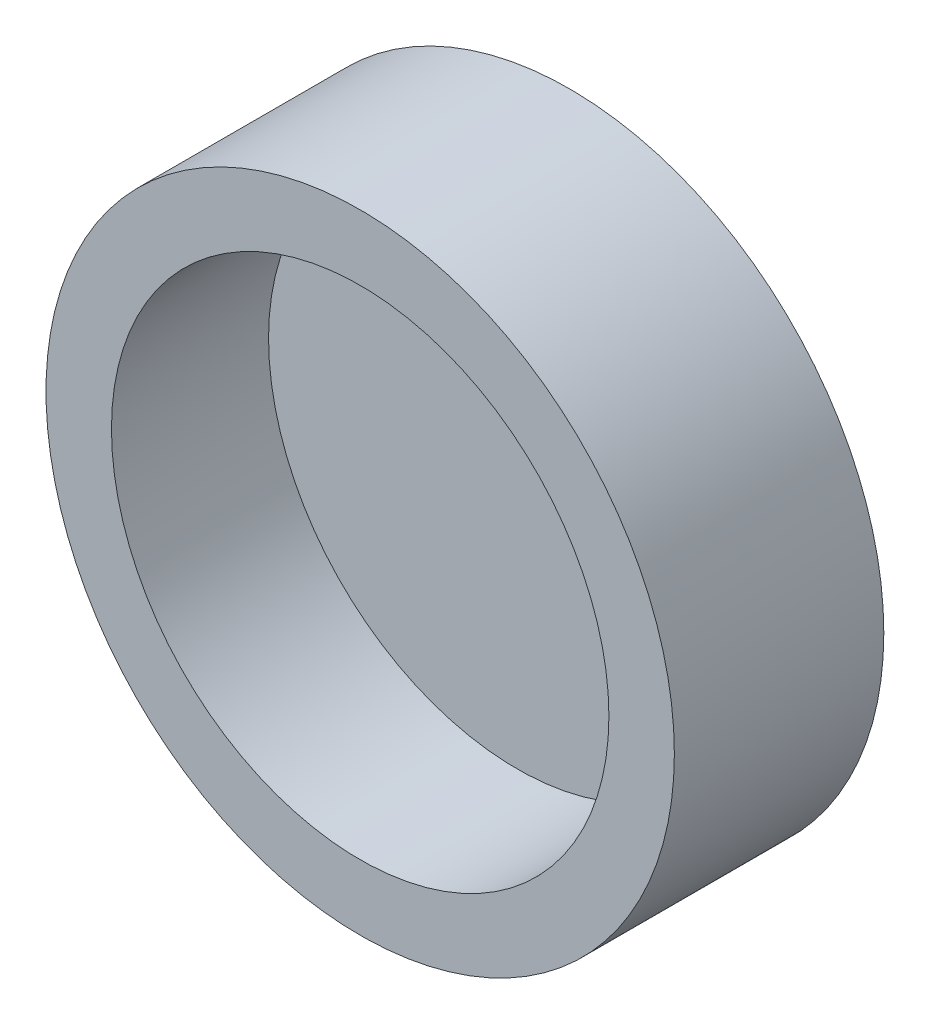
from build123d import *

# Parameters (mm, degrees)
SKETCH1_R           = 12
BOSS_EXTRUDE1_DEPTH = 8
SKETCH2_R           = 9.5
CUT_EXTRUDE1_DEPTH  = 6


with BuildPart() as part:
    # Sketch1 → Boss-Extrude1 (new body)
    with BuildSketch(Plane.XY):
        Circle(SKETCH1_R)
    extrude(amount=BOSS_EXTRUDE1_DEPTH)

    # Sketch2 → Cut-Extrude1 (cut)
    with BuildSketch(Plane.XY.offset(8)):
        Circle(SKETCH2_R)
    extrude(amount=-CUT_EXTRUDE1_DEPTH, mode=Mode.SUBTRACT)


solid = part.part
